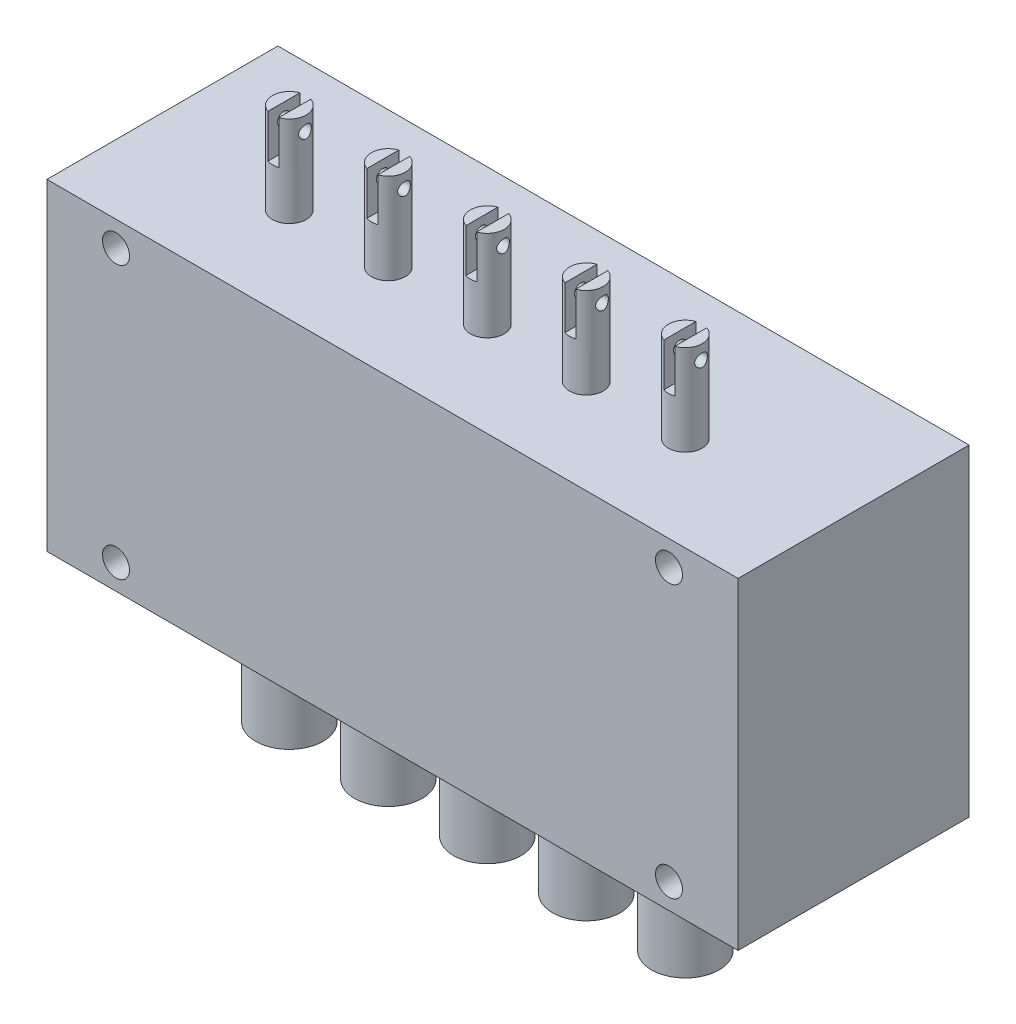
from build123d import *

# Parameters (mm, degrees)
SKETCH1_W            = 266
SKETCH1_H            = 124
BOSS_EXTRUDE1_DEPTH  = 88.9
SKETCH2_R            = 5.2
CUT_EXTRUDE1_DEPTH   = 88.9
LPATTERN1_COUNT      = 52
LPATTERN1_PITCH      = 212.8
LPATTERN1_COUNT_DIR2 = 2
LPATTERN1_PITCH_DIR2 = 104.7
SKETCH3_R            = 6.5
BOSS_EXTRUDE2_DEPTH  = 34.85
LPATTERN2_COUNT      = 5
LPATTERN2_PITCH      = 38.1
SKETCH6_R            = 13
BOSS_EXTRUDE3_DEPTH  = 46.65
LPATTERN5_COUNT      = 5
LPATTERN5_PITCH      = 38.1
SKETCH7_R            = 2.44
CUT_EXTRUDE2_DEPTH   = 301.772393181
CUT_EXTRUDE3_DEPTH   = 16.6
LPATTERN6_COUNT      = 5
LPATTERN6_PITCH      = 38.1


with BuildPart() as part:
    # Sketch1 → Boss-Extrude1 (new body)
    with BuildSketch(Plane.XY):
        Rectangle(SKETCH1_W, SKETCH1_H)
    extrude(amount=BOSS_EXTRUDE1_DEPTH)

    # Sketch2 → Cut-Extrude1 (cut)
    with BuildSketch(Plane.XY.offset(88.9)):
        with Locations((-106.4, 52.35)):
            Circle(SKETCH2_R)
    cut_extrude1 = extrude(amount=-CUT_EXTRUDE1_DEPTH, mode=Mode.SUBTRACT)

    # LPattern1: Cut-Extrude1 52 × 2
    with Locations(*[(i * LPATTERN1_PITCH, -j * LPATTERN1_PITCH_DIR2, 0) for i in range(LPATTERN1_COUNT) for j in range(LPATTERN1_COUNT_DIR2) if (i, j) != (0, 0)]):
        add(cut_extrude1, mode=Mode.SUBTRACT)

    # Sketch3 → Boss-Extrude2 (add)
    with BuildSketch(Plane(origin=(0, 62, 0), x_dir=(1, 0, 0), z_dir=(0, 1, 0))):
        with Locations(Location((-76.2, -52.4, 0), (0, 0, 90))):
            Circle(SKETCH3_R)
    boss_extrude2 = extrude(amount=BOSS_EXTRUDE2_DEPTH)

    # LPattern2: Boss-Extrude2 ×5
    with Locations(*[(i * LPATTERN2_PITCH, 0, 0) for i in range(1, LPATTERN2_COUNT)]):
        add(boss_extrude2)

    # Sketch6 → Boss-Extrude3 (add)
    with BuildSketch(Plane.XZ.offset(62)):
        with Locations(Location((-76.2, 52.4, 0), (0, 0, 90))):
            Circle(SKETCH6_R)
    boss_extrude3 = extrude(amount=BOSS_EXTRUDE3_DEPTH)

    # LPattern5: Boss-Extrude3 ×5
    with Locations(*[(i * LPATTERN5_PITCH, 0, 0) for i in range(1, LPATTERN5_COUNT)]):
        add(boss_extrude3)

    # Sketch7 → Cut-Extrude2 (cut, through all)
    with BuildSketch(Plane.ZY.offset(133)):
        with Locations((52.4, 91.35)):
            Circle(SKETCH7_R)
    extrude(amount=-CUT_EXTRUDE2_DEPTH, mode=Mode.SUBTRACT)

    # Sketch8 → Cut-Extrude3 (cut)
    with BuildSketch(Plane(origin=(0, 96.85, 0), x_dir=(1, 0, 0), z_dir=(0, 1, 0))):
        with BuildLine():
            Line((-78.3, -45.72242559), (-78.3, -59.07757441))
            ThreePointArc((-78.3, -59.07757441), (-76.2, -59.4), (-74.1, -59.07757441))
            Line((-74.1, -59.07757441), (-74.1, -45.72242559))
            ThreePointArc((-74.1, -45.72242559), (-76.2, -45.4), (-78.3, -45.72242559))
        make_face()
    cut_extrude3 = extrude(amount=-CUT_EXTRUDE3_DEPTH, mode=Mode.SUBTRACT)

    # LPattern6: Cut-Extrude3 ×5
    with Locations(*[(i * LPATTERN6_PITCH, 0, 0) for i in range(1, LPATTERN6_COUNT)]):
        add(cut_extrude3, mode=Mode.SUBTRACT)


solid = part.part
